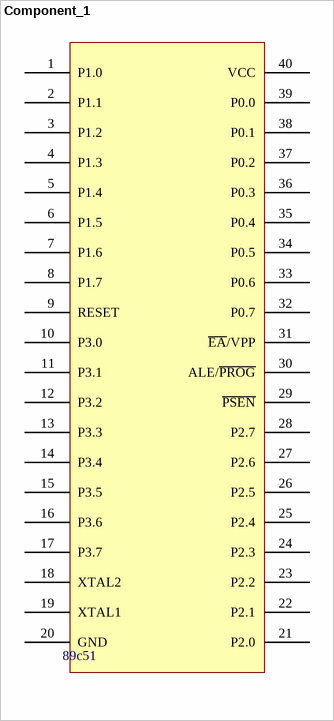
[diagram p0: symbol Component_1]
# Altium schematic symbol library MISC89340-4.SchLib: 1 symbol
Pins are listed as number, name and electrical type; pins without a type are passive.


## Component_1
designator 89c51
footprint 89c51
pins: 1 P1.0, 2 P1.1, 3 P1.2, 4 P1.3, 5 P1.4, 6 P1.5, 7 P1.6, 8 P1.7, 9 RESET, 10 P3.0, 11 P3.1, 12 P3.2, 13 P3.3, 14 P3.4, 15 P3.5, 16 P3.6, 17 P3.7, 18 XTAL2, 19 XTAL1, 20 GND, 21 P2.0, 22 P2.1, 23 P2.2, 24 P2.3, 25 P2.4, 26 P2.5, 27 P2.6, 28 P2.7, 29 ~{PSEN}, 30 ALE/~{PROG}, 31 ~{EA}/VPP, 32 P0.7, 33 P0.6, 34 P0.5, 35 P0.4, 36 P0.3, 37 P0.2, 38 P0.1, 39 P0.0, 40 VCC